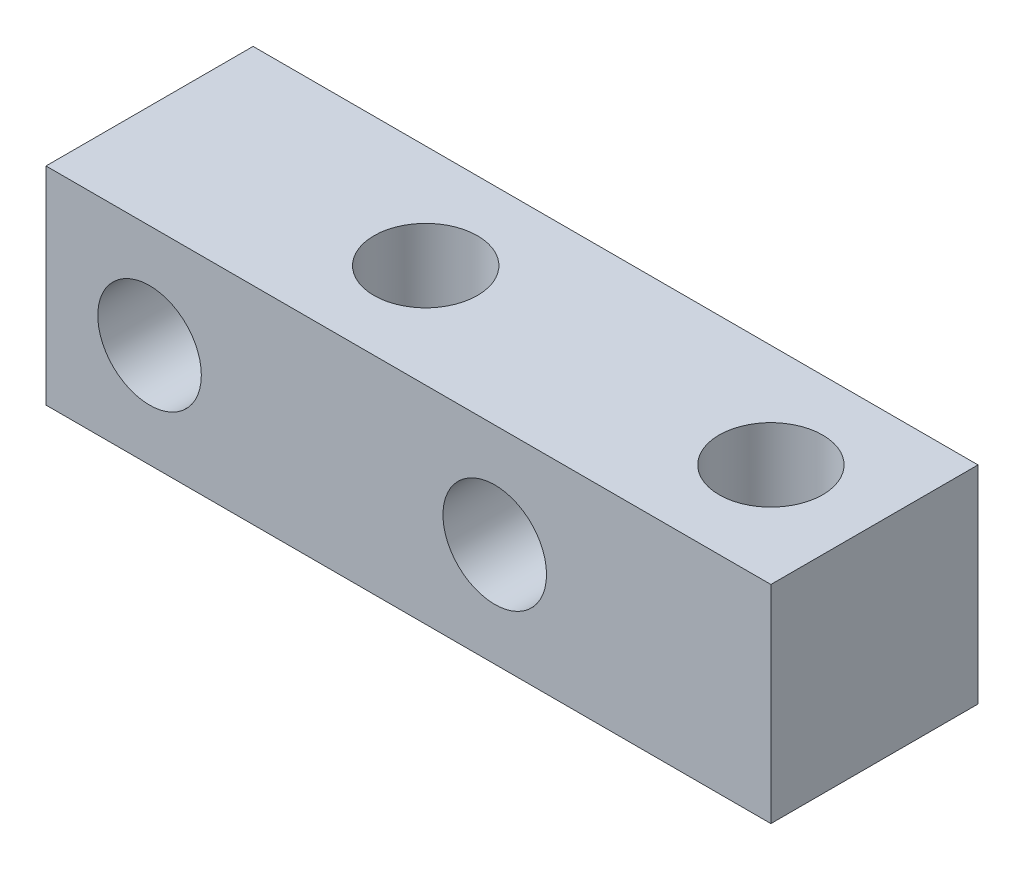
from build123d import *

# Parameters (mm, degrees)
SKETCH_1_W               = 21
SKETCH_1_H               = 6
SKETCH_1_R               = 1.5
EXTRUDE_1_DEPTH          = 6
CUT_EXTRUDE_1_DEPTH      = 23.649503306
CUT_EXTRUDE_1_DEPTH_BACK = 23.649503306
SKETCH_2_R               = 1.5


with BuildPart() as part:
    # 草图1 → 凸台-拉伸1 (new body)
    with BuildSketch(Plane.XY):
        with Locations((10.5, 3)):
            Rectangle(SKETCH_1_W, SKETCH_1_H)
        with Locations((3, 3)):
            Circle(SKETCH_1_R, mode=Mode.SUBTRACT)
        with Locations((13, 3)):
            Circle(SKETCH_1_R, mode=Mode.SUBTRACT)
    extrude(amount=EXTRUDE_1_DEPTH)

    # 草图2 → 切除-拉伸1 (cut, two sides: drawn at the far end of the back side and taken through both)
    with BuildSketch(Plane(origin=(0, 6, 0), x_dir=(1, 0, 0), z_dir=(0, 1, 0)).offset(-CUT_EXTRUDE_1_DEPTH_BACK)):
        with Locations(Location((8, -3, 0), (0, 0, 270))):
            Circle(SKETCH_2_R)
        with Locations(Location((18, -3, 0), (0, 0, 270))):
            Circle(SKETCH_2_R)
    extrude(amount=CUT_EXTRUDE_1_DEPTH + CUT_EXTRUDE_1_DEPTH_BACK, mode=Mode.SUBTRACT)


solid = part.part
